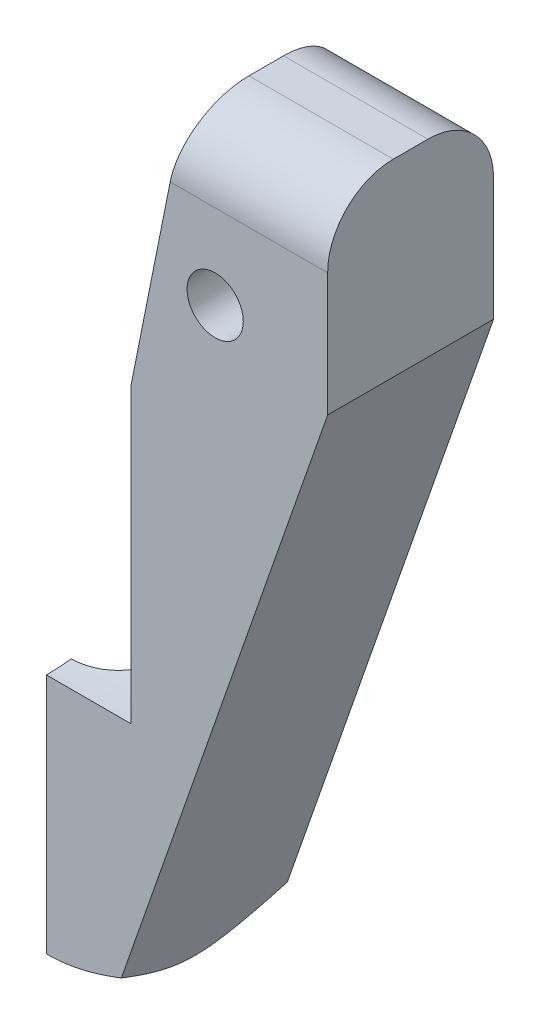
from build123d import *

# Parameters (mm, degrees)
SKETCH1_R                      = 3
BOSS_EXTRUDE2_DEPTH            = 17.7
CUT_EXTRUDE1_REACH             = 94.786
CUT_EXTRUDE1_DIRECTION_2_REACH = 94.786
SKETCH6_RX                     = 12.258033
SKETCH6_RY                     = 6.491927
CUT_EXTRUDE2_DEPTH             = 48.7
SKETCH7_R                      = 6.19409
CUT_EXTRUDE3_DEPTH             = 60.7
SKETCH8_R                      = 4
CUT_EXTRUDE4_DEPTH             = 48
FILLET1_R                      = 7
SKETCH10_OUTSIDE_W             = 249.546
SKETCH10_OUTSIDE_H             = 207.246
SKETCH10_OUTSIDE_R             = 7
CUT_EXTRUDE5_DEPTH             = 48
CUT_EXTRUDE5_TAPER             = 60
CUT_EXTRUDE8_DEPTH             = 44


with BuildPart() as part:
    # Sketch1 → Boss-Extrude2 (new body)
    with BuildSketch(Plane.XY):
        with BuildLine():
            Line((39, -51.503555), (34.837666, -51.503555))
            Line((34.837666, -51.503555), (25.162334, -51.503555))
            Line((25.162334, -51.503555), (21, -51.503555))
            Line((21, -51.503555), (21, -28.6))
            Line((21, -28.6), (15.376404, 0))
            Line((15.376404, 0), (0, 0))
            Line((0, 0), (0, -20.136364))
            Line((0, -20.136364), (21.048788, -80.412439))
            add(Edge.make_bspline(
                [(21.669142, -82.188906), (21.466678, -81.609123), (21.259066, -81.014599), (21.048788, -80.412439)],
                knots=[0.75, 0.75, 0.75, 0.75, 1, 1, 1, 1], degree=3))
            add(Edge.make_bspline(
                [(22.255532, -83.868113), (22.06924, -83.334643), (21.871606, -82.768689), (21.669142, -82.188906)],
                knots=[0.5, 0.5, 0.5, 0.5, 0.75, 0.75, 0.75, 0.75], degree=3))
            add(Edge.make_bspline(
                [(22.524034, -84.637007), (22.439154, -84.393941), (22.348677, -84.134848), (22.255532, -83.868113)],
                knots=[0.375, 0.375, 0.375, 0.375, 0.5, 0.5, 0.5, 0.5], degree=3))
            add(Edge.make_bspline(
                [(22.758263, -85.307753), (22.688292, -85.107381), (22.608914, -84.880073), (22.524034, -84.637007)],
                knots=[0.25, 0.25, 0.25, 0.25, 0.375, 0.375, 0.375, 0.375], degree=3))
            add(Edge.make_bspline(
                [(22.855261, -85.585519), (22.825847, -85.50129), (22.793248, -85.407938), (22.758263, -85.307753)],
                knots=[0.1875, 0.1875, 0.1875, 0.1875, 0.25, 0.25, 0.25, 0.25], degree=3))
            add(Edge.make_bspline(
                [(22.932474, -85.806631), (22.910958, -85.745015), (22.884674, -85.669748), (22.855261, -85.585519)],
                knots=[0.125, 0.125, 0.125, 0.125, 0.1875, 0.1875, 0.1875, 0.1875], degree=3))
            add(Edge.make_bspline(
                [(23, -86), (22.975508, -85.929864), (22.932474, -85.806631)],
                knots=[0, 0, 0, 0.125, 0.125, 0.125], degree=2))
            Line((23, -86), (37, -86))
            add(Edge.make_bspline(
                [(37.068167, -85.804796), (37.025162, -85.927946), (37, -86)],
                knots=[0.875, 0.875, 0.875, 1, 1, 1], degree=2))
            add(Edge.make_bspline(
                [(37.242328, -85.306061), (37.171936, -85.507639), (37.111171, -85.681646), (37.068167, -85.804796)],
                knots=[0.75, 0.75, 0.75, 0.75, 0.875, 0.875, 0.875, 0.875], degree=3))
            add(Edge.make_bspline(
                [(37.47673, -84.63482), (37.392157, -84.877005), (37.31272, -85.104482), (37.242328, -85.306061)],
                knots=[0.625, 0.625, 0.625, 0.625, 0.75, 0.75, 0.75, 0.75], degree=3))
            add(Edge.make_bspline(
                [(37.744144, -83.869041), (37.651111, -84.135454), (37.561302, -84.392634), (37.47673, -84.63482)],
                knots=[0.5, 0.5, 0.5, 0.5, 0.625, 0.625, 0.625, 0.625], degree=3))
            add(Edge.make_bspline(
                [(38.330881, -82.18884), (38.128355, -82.768803), (37.930211, -83.336215), (37.744144, -83.869041)],
                knots=[0.25, 0.25, 0.25, 0.25, 0.5, 0.5, 0.5, 0.5], degree=3))
            add(Edge.make_bspline(
                [(38.951212, -80.412439), (38.741, -81.014409), (38.533408, -81.608878), (38.330881, -82.18884)],
                knots=[0, 0, 0, 0, 0.25, 0.25, 0.25, 0.25], degree=3))
            Line((38.951212, -80.412439), (60, -20.136364))
            Line((60, -20.136364), (60, 0))
            Line((60, 0), (44.6, 0))
            Line((44.6, 0), (39, -28))
            Line((39, -28), (39, -51.503555))
        make_face()
        with Locations((48, -16)):
            Circle(SKETCH1_R, mode=Mode.SUBTRACT)
        with Locations((12, -16)):
            Circle(SKETCH1_R, mode=Mode.SUBTRACT)
    extrude(amount=BOSS_EXTRUDE2_DEPTH)

    # Sketch2 → Cut-Revolve2 (revolve, cut)
    with BuildSketch(Plane.ZY.offset(-30), mode=Mode.PRIVATE) as cut_revolve2_sk:
        with BuildLine():
            ThreePointArc((11.5, -81.75), (11.729241, -80.820262), (12.364412, -80.103659))
            ThreePointArc((12.364412, -80.103659), (14.333443, -77.882187), (15.04409, -75))
            Line((15.04409, -75), (15.04409, -57.48))
            Line((15.04409, -57.48), (8.85, -57.48))
            Line((8.85, -57.48), (8.85, -86))
            Line((8.85, -86), (11.5, -86))
            Line((11.5, -86), (11.5, -81.75))
        make_face()
    revolve(cut_revolve2_sk.sketch.rotate(Axis((30, -86, 8.85), (0, 1, 0)), 180), axis=Axis((30, -86, 8.85), (0, 1, 0)), mode=Mode.SUBTRACT)

    # Cut-Extrude1: up to this face of the body (flat: up to its plane)
    cut_extrude1_end = Plane(part.part.faces().sort_by_distance((39, -39.751777, 8.85))[0])
    # Sketch3 → Cut-Extrude1 (cut, up to the picked face)
    with BuildSketch(Plane.ZY.offset(-30), mode=Mode.PRIVATE) as cut_extrude1_sk1:
        with BuildLine():
            Line((0, -51.503555), (17.7, -51.503555))
            Line((17.7, -51.503555), (17.7, -59.152297))
            add(Edge.make_bspline(
                [(17.7, -59.152297), (7.335394, -59.008853), (0, -51.503555)],
                knots=[0, 0, 0, 1, 1, 1], degree=2))
        make_face()
    cut_extrude1_tool1 = split(extrude(cut_extrude1_sk1.sketch, amount=-CUT_EXTRUDE1_REACH, mode=Mode.PRIVATE), bisect_by=cut_extrude1_end, keep=Keep.BOTH, mode=Mode.PRIVATE)
    add(cut_extrude1_tool1.solids().sort_by(Axis((30, -54.604638, 10.907898), (1, 0, 0)))[0], mode=Mode.SUBTRACT)

    # Cut-Extrude1 direction 2: up to this face of the body (flat: up to its plane)
    cut_extrude1_direction_2_end = Plane(part.part.faces().sort_by_distance((21, -40.051777, 8.85))[0])
    # Sketch3 → Cut-Extrude1 direction 2 (cut, up to the picked face)
    with BuildSketch(Plane.ZY.offset(-30), mode=Mode.PRIVATE) as cut_extrude1_direction_2_sk1:
        with BuildLine():
            Line((0, -51.503555), (17.7, -51.503555))
            Line((17.7, -51.503555), (17.7, -59.152297))
            add(Edge.make_bspline(
                [(17.7, -59.152297), (7.335394, -59.008853), (0, -51.503555)],
                knots=[0, 0, 0, 1, 1, 1], degree=2))
        make_face()
    cut_extrude1_direction_2_tool1 = split(extrude(cut_extrude1_direction_2_sk1.sketch, amount=CUT_EXTRUDE1_DIRECTION_2_REACH, mode=Mode.PRIVATE), bisect_by=cut_extrude1_direction_2_end, keep=Keep.BOTH, mode=Mode.PRIVATE)
    add(cut_extrude1_direction_2_tool1.solids().sort_by(Axis((30, -54.604638, 10.907898), (-1, 0, 0)))[0], mode=Mode.SUBTRACT)

    # Sketch6 → Cut-Extrude2 (cut)
    with BuildSketch(Plane(origin=(0, 0, 8.85), x_dir=(-1, 0, 0), z_dir=(0, 0, -1))):
        with Locations(Location((-30, -47.968312), (0, 0, 90))):
            Ellipse(SKETCH6_RX, SKETCH6_RY)
    extrude(amount=CUT_EXTRUDE2_DEPTH, mode=Mode.SUBTRACT)

    # Sketch7 → Cut-Extrude3 (cut)
    with BuildSketch(Plane(origin=(0, 0, 0), x_dir=(1, 0, 0), z_dir=(0, 1, 0))):
        with Locations(Location((30, -8.85, 0), (0, 0, 90))):
            Circle(SKETCH7_R)
    extrude(amount=-CUT_EXTRUDE3_DEPTH, mode=Mode.SUBTRACT)

    # Sketch8 → Cut-Extrude4 (cut)
    with BuildSketch(Plane.ZY.offset(-6)):
        with Locations((8.85, -5)):
            Circle(SKETCH8_R)
    extrude(amount=-CUT_EXTRUDE4_DEPTH, mode=Mode.SUBTRACT)

    # Fillet1
    fillet1_edges = [part.edges().sort_by_distance(p)[0] for p in [
        (7.688202, 0, 17.7),
        (52.3, 0, 0),
        (7.688202, 0, 0),
        (52.3, 0, 17.7),
    ]]
    fillet(fillet1_edges, radius=FILLET1_R)

    # Sketch10 outside → Cut-Extrude5 (cut)
    with BuildSketch(Plane.XZ.offset(86)):
        with Locations((30, 8.85)):
            Rectangle(SKETCH10_OUTSIDE_W, SKETCH10_OUTSIDE_H)
        with Locations((30, 8.85)):
            Circle(SKETCH10_OUTSIDE_R, mode=Mode.SUBTRACT)
    extrude(amount=-CUT_EXTRUDE5_DEPTH, taper=CUT_EXTRUDE5_TAPER, mode=Mode.SUBTRACT)

    # Sketch12 → Cut-Extrude8 (cut)
    with BuildSketch(Plane.XY.offset(17.7)):
        Polygon((30, -86), (30, 13.730719), (-24.441977, 10.861444), (-8.282064, -99.477746), align=None)
    extrude(amount=-CUT_EXTRUDE8_DEPTH, mode=Mode.SUBTRACT)


solid = part.part
